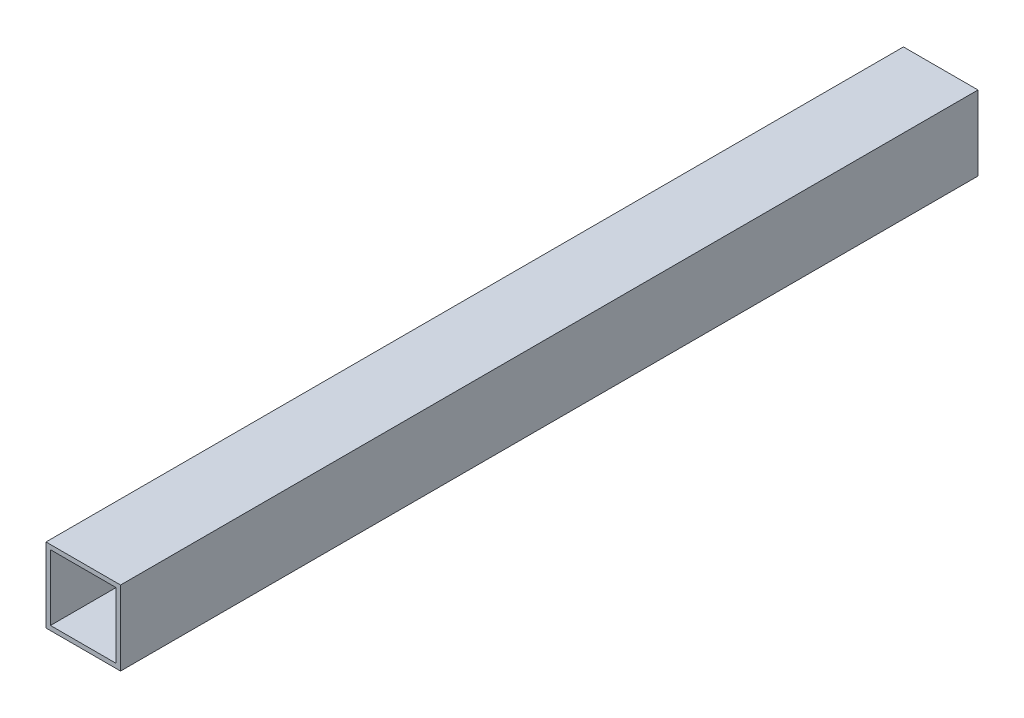
from build123d import *

# Parameters (mm, degrees)
SKETCH_1_W          = 50
SKETCH_1_H          = 50
SKETCH_1_W_2        = 44
SKETCH_1_H_2        = 44
EXTRUDE_1_DEPTH     = 600
SKETCH_2_W          = 50
SKETCH_2_H          = 50
SKETCH_2_W_2        = 44
SKETCH_2_H_2        = 44
CUT_EXTRUDE_1_DEPTH = 25


with BuildPart() as part:
    # 草图1 → 凸台-拉伸1 (new body)
    with BuildSketch(Plane.XY):
        with Locations((25, 25)):
            Rectangle(SKETCH_1_W, SKETCH_1_H)
        with Locations((25, 25)):
            Rectangle(SKETCH_1_W_2, SKETCH_1_H_2, mode=Mode.SUBTRACT)
    extrude(amount=EXTRUDE_1_DEPTH)

    # 草图2 → 切除-拉伸1 (cut)
    with BuildSketch(Plane.XY.offset(600)):
        with Locations((25, 25)):
            Rectangle(SKETCH_2_W, SKETCH_2_H)
        with Locations((25, 25)):
            Rectangle(SKETCH_2_W_2, SKETCH_2_H_2, mode=Mode.SUBTRACT)
    extrude(amount=-CUT_EXTRUDE_1_DEPTH, mode=Mode.SUBTRACT)


solid = part.part
